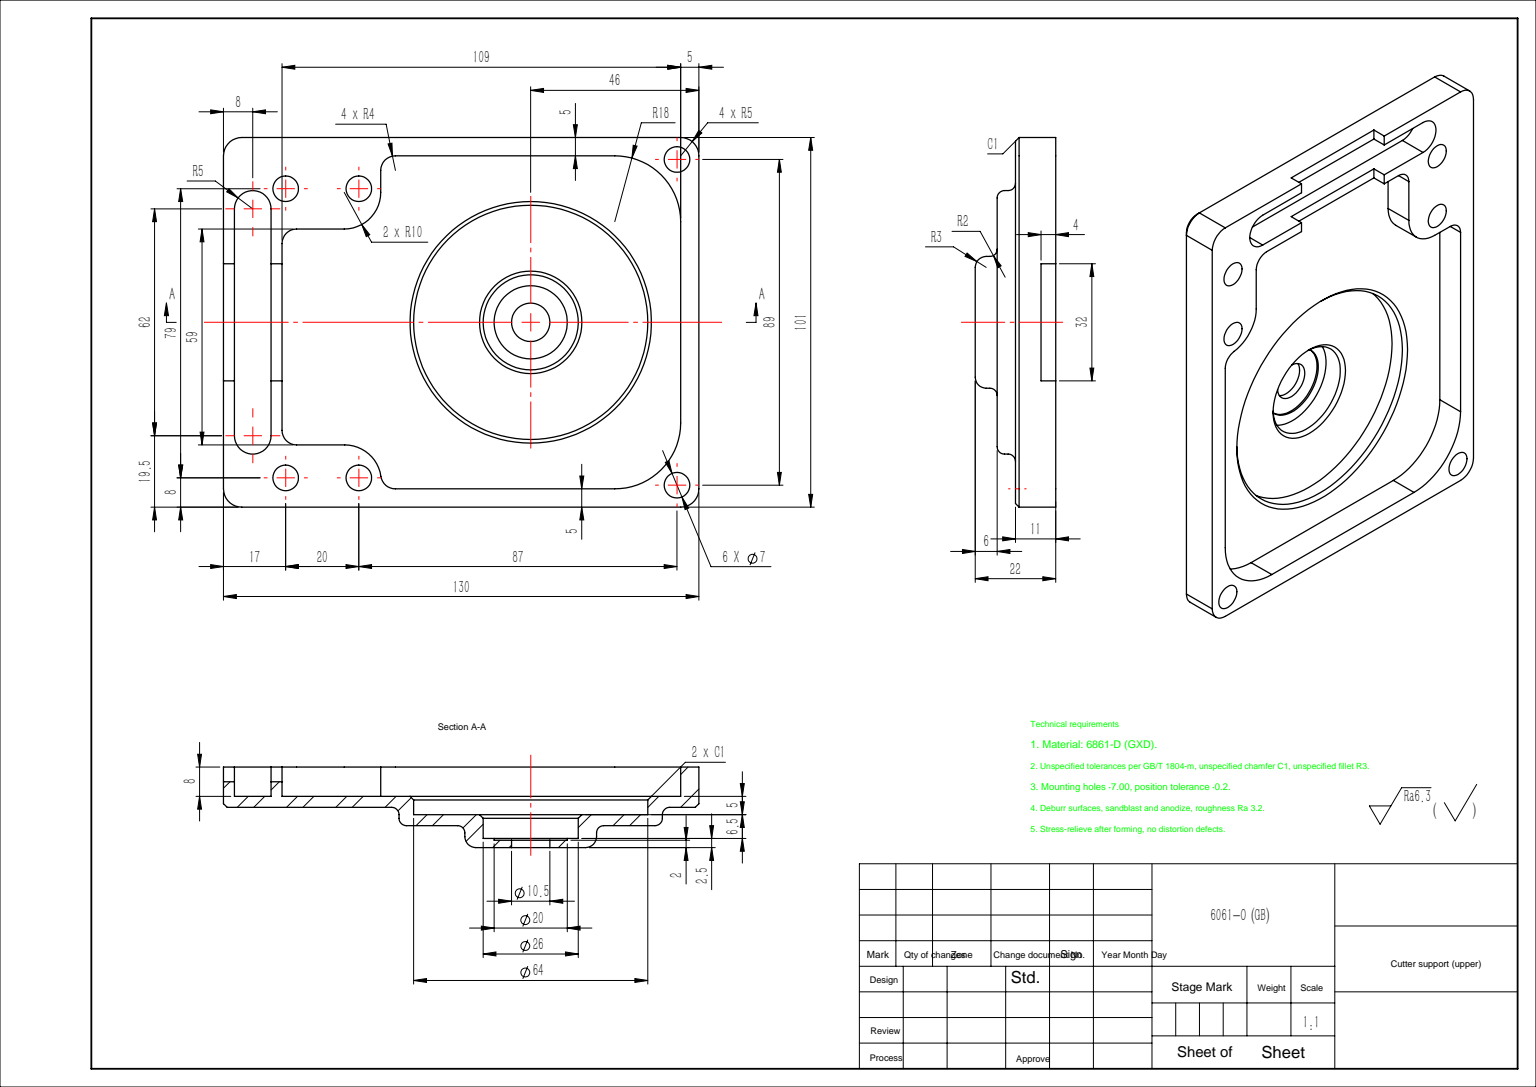
SolidWorks part; units mm, degrees
material "6061-O (GB)"
ref_plane "前视基准面" through (0, 0, 0) normal (0, 0, 1) x (1, 0, 0)
ref_plane "上视基准面" through (0, 0, 0) normal (0, 1, 0) x (1, 0, 0)
ref_plane "右视基准面" through (0, 0, 0) normal (1, 0, 0) x (0, 0, -1)
ref_plane "基准面4" through (1263, 0, 0) normal (1, 0, 0) x (0, 0, -1)
sketch "草图1" plane through (1263, 0, 0) normal (1, 0, 0) x (0, 0, -1)
  line L0 (39.5, 58.4) -> (-61.5, 58.4)
  line L1 (-61.5, 58.4) -> (-61.5, -71.6)
  line L2 (-61.5, -71.6) -> (39.5, -71.6)
  line L3 (39.5, -71.6) -> (39.5, 58.4)
extrude "凸台-拉伸1" add sketch "草图1" against normal blind 11
sketch "草图2" plane through (1263, 0, 0) normal (1, 0, 0) x (0, 0, -1)
  line L0 (14.5, 42.4) -> (-44.5, 42.4)
  line L1 (-44.5, 42.4) -> (-44.5, 25.2564)
  line L2 (-56.5, 15.4584) -> (-56.5, -48.6)
  line L3 (-38.5, -66.6) -> (16.5, -66.6)
  line L4 (34.5, -48.6) -> (34.5, 15.4)
  line L5 (34.5, 15.4) -> (14.5, 15.4)
  line L6 (14.5, 15.4) -> (14.5, 42.4)
  arc A0 (-44.5, 25.2564) -> (-56.5, 15.4584) centre (-54.5, 25.2564) cw
  arc A1 (-56.5, -48.6) -> (-38.5, -66.6) centre (-38.5, -48.6) ccw
  arc A2 (16.5, -66.6) -> (34.5, -48.6) centre (16.5, -48.6) ccw
extrude "切除-拉伸1" cut sketch "草图2" against normal blind 8
sketch "草图3" plane through (1263, 0, 0) normal (1, 0, 0) x (0, 0, -1)
  line L0 (20, 55.4) -> (-42, 55.4)
  line L1 (-42, 45.4) -> (20, 45.4)
  arc A0 (20, 45.4) -> (20, 55.4) centre (20, 50.4) ccw
  arc A1 (-42, 55.4) -> (-42, 45.4) centre (-42, 50.4) ccw
extrude "切除-拉伸2" cut sketch "草图3" against normal blind 8
sketch "草图4" plane through (0, 42.4, 0) normal (0, -1, 0) x (1, 0, 0)
  line L0 (1263, -5) -> (1263, 27)
  line L1 (1263, 27) -> (1259, 27)
  line L2 (1259, 27) -> (1259, -5)
  line L3 (1259, -5) -> (1263, -5)
extrude "切除-拉伸3" cut sketch "草图4" against normal up to next
sketch "草图5" plane through (0, 58.4, 0) normal (0, 1, 0) x (-1, 0, 0)
  line L0 (-1263, 27) -> (-1263, -5)
  line L1 (-1263, -5) -> (-1259, -5)
  line L2 (-1259, -5) -> (-1259, 27)
  line L3 (-1259, 27) -> (-1263, 27)
extrude "切除-拉伸4" cut sketch "草图5" against normal up to next
sketch "草图6" plane through (1252, 0, 0) normal (-1, 0, 0) x (0, 0, 1)
  circle A0 centre (11, -25.6) radius 36
extrude "凸台-拉伸2" add sketch "草图6" along normal blind 5
sketch "草图7" plane through (1247, 0, 0) normal (-1, 0, 0) x (0, 0, 1)
  circle A0 centre (11, -25.6) radius 18
extrude "凸台-拉伸3" add sketch "草图7" along normal blind 6
sketch "草图8" plane through (1255, 0, 0) normal (1, 0, 0) x (0, 0, -1)
  circle A0 centre (-11, -25.6) radius 32
extrude "切除-拉伸5" cut sketch "草图8" against normal blind 5
sketch "草图9" plane through (1250, 0, 0) normal (1, 0, 0) x (0, 0, -1)
  circle A0 centre (-11, -25.6) radius 13
extrude "切除-拉伸6" cut sketch "草图9" against normal blind 6.5
sketch "草图10" plane through (1243.5, 0, 0) normal (1, 0, 0) x (0, 0, -1)
  circle A0 centre (-11, -25.6) radius 10
extrude "切除-拉伸7" cut sketch "草图10" against normal blind 0.5
sketch "草图11" plane through (1241, 0, 0) normal (-1, 0, 0) x (0, 0, 1)
  circle A0 centre (11, -25.6) radius 5.25
extrude "切除-拉伸8" cut sketch "草图11" against normal through all
hole_wizard "Ø7.0 (7) 直径孔1" positions "草图13" profile "草图12" hole size "Ø7.0" standard "ANSI Metric"
sketch "草图13" plane through (1263, 0, 0) normal (1, 0, 0) x (0, 0, -1)
  point P0 (-55.5, -65.6)
  point P1 (33.5, -65.6)
  point P2 (25.5, 21.4)
  point P3 (25.5, 41.4)
  point P4 (-53.5, 41.4)
  point P5 (-53.5, 21.4)
sketch "草图12" plane through (1263, -65.6, 55.5) normal (0, 1, 0) x (0, 0, -1)
  line L0 (0, 0) -> (0, 22)
  line L1 (0, 22) -> (3.5, 22)
  line L2 (3.5, 22) -> (3.5, 0)
  line L5 (3.5, 0) -> (0, 0)
  line L11 (0, -6.35) -> (0, 107.95) construction
  dimension "通孔孔直径" = 7
  dimension "通孔孔深度" = 22
fillet "圆角1" radius 5 4 edges at (1257.5, 58.4, 61.5) (1257.5, 58.4, -39.5) (1257.5, -71.6, -39.5) (1257.5, -71.6, 61.5)
chamfer "倒角1" distance 1 angle 45 10 edges at (1252, -70.1355, -38.0355) (1252, -71.6, 11) (1252, -6.6, -39.5) (1252, -70.1355, 60.0355) (1252, 56.9355, -38.0355) (1252, -6.6, 61.5) (1252, 58.4, 11) (1252, 56.9355, 60.0355) (1250, -25.6, 24) (1255, -25.6, 43)
fillet "圆角2" radius 2 3 edges at (1247, -25.6, 29) (1252, -25.6, 47) (1247, -25.6, 47)
fillet "圆角3" radius 3 1 edges at (1241, -25.6, 29)
fillet "圆角4" radius 4 4 edges at (1259, 42.4, -14.5) (1259, 15.4, -34.5) (1259, 42.4, 44.5) (1259, 15.4584, 56.5)
fillet "圆角5" radius 10 1 edges at (1259, 15.4, -14.5)
